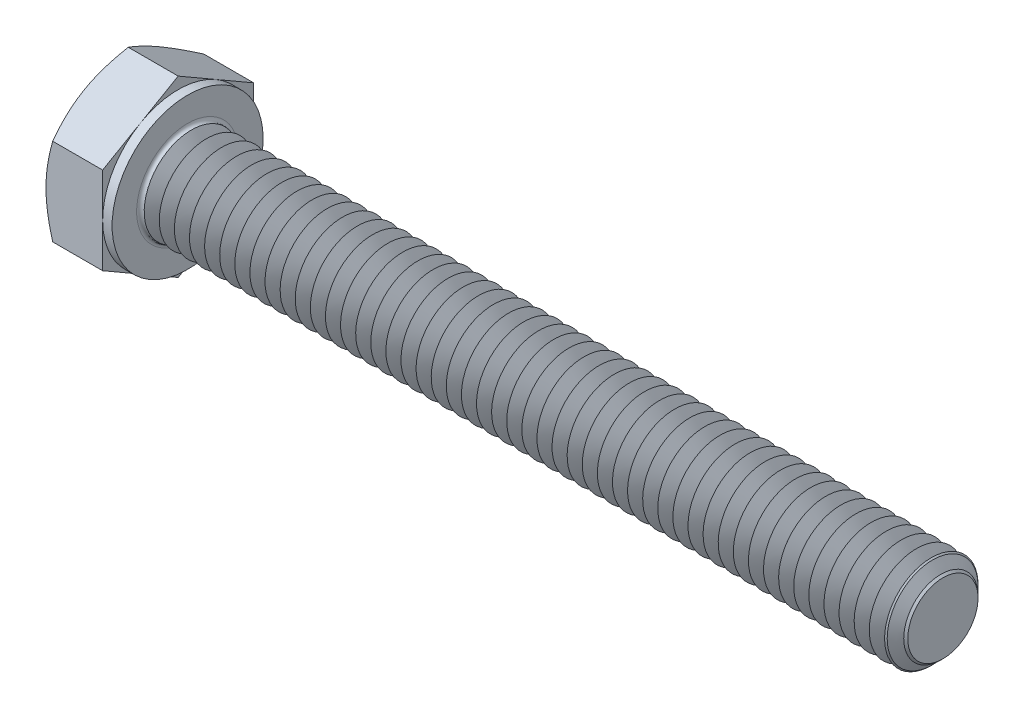
from build123d import *

# Parameters (mm, degrees)
BOSS_EXTRUDE_DEPTH = 3.5
SKETCH4_W          = 0.5
SKETCH4_H          = 10.618802154
CHAMFER_2_SIZE     = 0.64
FILLET_2_R         = 0.2
LPATTERN1_COUNT    = 50
LPATTERN1_PITCH    = 0.8


with BuildPart() as part:
    # Sketch1 → Boss-Extrude (new body)
    with BuildSketch(Plane(origin=(0, 0, 0), x_dir=(0, 0, -1), z_dir=(1, 0, 0))):
        Polygon((4, 2.309401077), (4, -2.309401077), (0, -4.618802154), (-4, -2.309401077), (-4, 2.309401077), (0, 4.618802154), align=None)
    extrude(amount=BOSS_EXTRUDE_DEPTH)

    # Sketch2 → Boss-Revolve1 (revolve)
    with BuildSketch(Plane.XY, mode=Mode.PRIVATE) as boss_revolve1_sk:
        Polygon((0, 0), (43.5, 0), (43.5, 1.8072), (43.5, 2.5), (0, 2.5), align=None)
    revolve(boss_revolve1_sk.sketch.rotate(Axis((0, 0, 0), (1, 0, 0)), 90), axis=Axis((0, 0, 0), (1, 0, 0)))

    # Sketch3 → Cut-Revolve1 (revolve, cut)
    with BuildSketch(Plane.XY):
        Polygon((0, 4), (3.244016936, 9.618802154), (3.244016936, 14.618802154), (-10, 14.618802154), (-10, 4), align=None)
    revolve(axis=Axis((0, 0, 0), (1, 0, 0)), mode=Mode.SUBTRACT)

    # Sketch5 → Cut-Revolve2 (revolve, cut)
    with BuildSketch(Plane.XY):
        Polygon((3.5, 4), (0.255983064, 9.618802154), (0.255983064, 14.618802154), (10.255983064, 14.618802154), (10.255983064, 4), align=None)
    revolve(axis=Axis((0, 0, 0), (1, 0, 0)), mode=Mode.SUBTRACT)

    # Sketch4 → Cut-Revolve3 (revolve, cut)
    with BuildSketch(Plane.XY, mode=Mode.PRIVATE) as cut_revolve3_sk:
        with Locations((3.25, 9.309401077)):
            Rectangle(SKETCH4_W, SKETCH4_H)
    revolve(cut_revolve3_sk.sketch.rotate(Axis((0, 0, 0), (1, 0, 0)), 270), axis=Axis((0, 0, 0), (1, 0, 0)), mode=Mode.SUBTRACT)

    # Chamfer 2
    chamfer_2_edges = [part.edges().sort_by_distance(p)[0] for p in [
        (43.5, 0, -2.5),
    ]]
    chamfer(chamfer_2_edges, length=CHAMFER_2_SIZE)

    # Fillet 2
    fillet_2_edges = [part.edges().sort_by_distance(p)[0] for p in [
        (3.5, 0, -2.5),
    ]]
    fillet(fillet_2_edges, radius=FILLET_2_R)

    # Sketch6 → Cut-Revolve4 (revolve, cut)
    with BuildSketch(Plane.XY):
        Polygon((4.099988266, -1.8072), (3.7, -2.5), (3.7, -3.125), (4.499976533, -3.125), (4.499976533, -2.5), align=None)
    cut_revolve4 = revolve(axis=Axis((-3.175, 0, 0), (1, 0, 0)), mode=Mode.SUBTRACT)

    # LPattern1: Cut-Revolve4 ×50
    with Locations(*[(i * LPATTERN1_PITCH, 0, 0) for i in range(1, LPATTERN1_COUNT)]):
        add(cut_revolve4, mode=Mode.SUBTRACT)


solid = part.part
